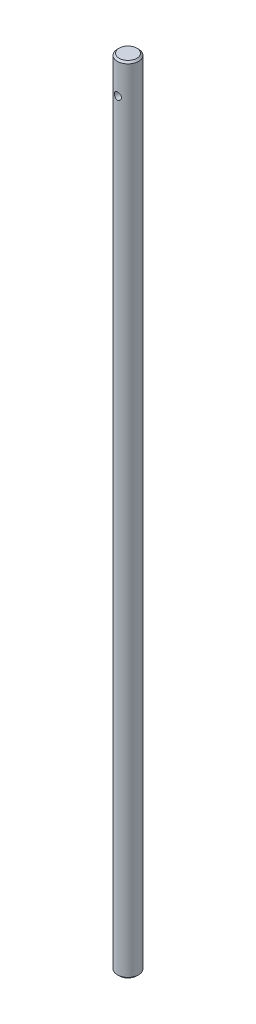
from build123d import *

# Parameters (mm, degrees)
SKETCH1_R               = 6
BOSS_EXTRUDE1_DEPTH     = 225
CHAMFER1_SIZE           = 1
CUT_EXTRUDE1_DEPTH      = 226.159943152
CUT_EXTRUDE1_DEPTH_BACK = 226.159943152
SKETCH2_R               = 2


with BuildPart() as part:
    # Sketch1 → Boss-Extrude1 (new, symmetric)
    with BuildSketch(Plane(origin=(0, 0, 0), x_dir=(1, 0, 0), z_dir=(0, 1, 0))):
        with Locations(Location((0, 0, 0), (0, 0, 270))):
            Circle(SKETCH1_R)
    extrude(amount=BOSS_EXTRUDE1_DEPTH, both=True)

    # Chamfer1
    chamfer1_edges = [part.edges().sort_by_distance(p)[0] for p in [
        (0, -225, -6),
        (0, 225, -6),
    ]]
    chamfer(chamfer1_edges, length=CHAMFER1_SIZE)

    # Sketch2 → Cut-Extrude1 (cut, two sides: drawn at the far end of the back side and taken through both)
    with BuildSketch(Plane.XY.offset(-CUT_EXTRUDE1_DEPTH_BACK)):
        with Locations(Location((0, 207, 0), (0, 0, 89.999999987))):
            Circle(SKETCH2_R)
    extrude(amount=CUT_EXTRUDE1_DEPTH + CUT_EXTRUDE1_DEPTH_BACK, mode=Mode.SUBTRACT)


solid = part.part
